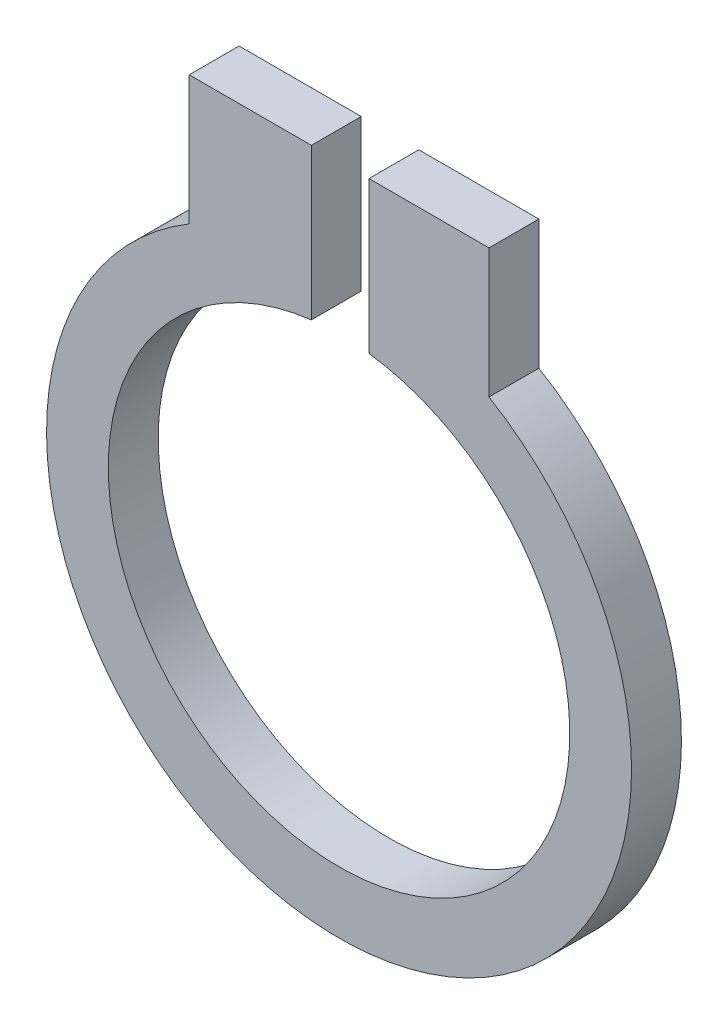
from build123d import *

# Parameters (mm, degrees)
BOSS_EXTRUDE1_DEPTH = 0.8


with BuildPart() as part:
    # Sketch1 → Boss-Extrude1 (new body)
    with BuildSketch(Plane.XY):
        with BuildLine():
            Line((-0.44416607, 3.673243322), (-0.44416607, 6.097784133))
            Line((-0.44416607, 6.097784133), (-2.402419126, 6.097784133))
            Line((-2.402419126, 6.097784133), (-2.402419126, 4.027962555))
            ThreePointArc((-2.402419126, 4.027962555), (-0.000948808, -4.689999904), (2.404048678, 4.026990186))
            Line((2.404048678, 4.026990186), (2.404048678, 6.097784133))
            Line((2.404048678, 6.097784133), (0.479079413, 6.097784133))
            Line((0.479079413, 6.097784133), (0.479079413, 3.668853079))
            ThreePointArc((0.479079413, 3.668853079), (-0.017594145, -3.699958168), (-0.44416607, 3.673243322))
        make_face()
    extrude(amount=BOSS_EXTRUDE1_DEPTH)


solid = part.part
